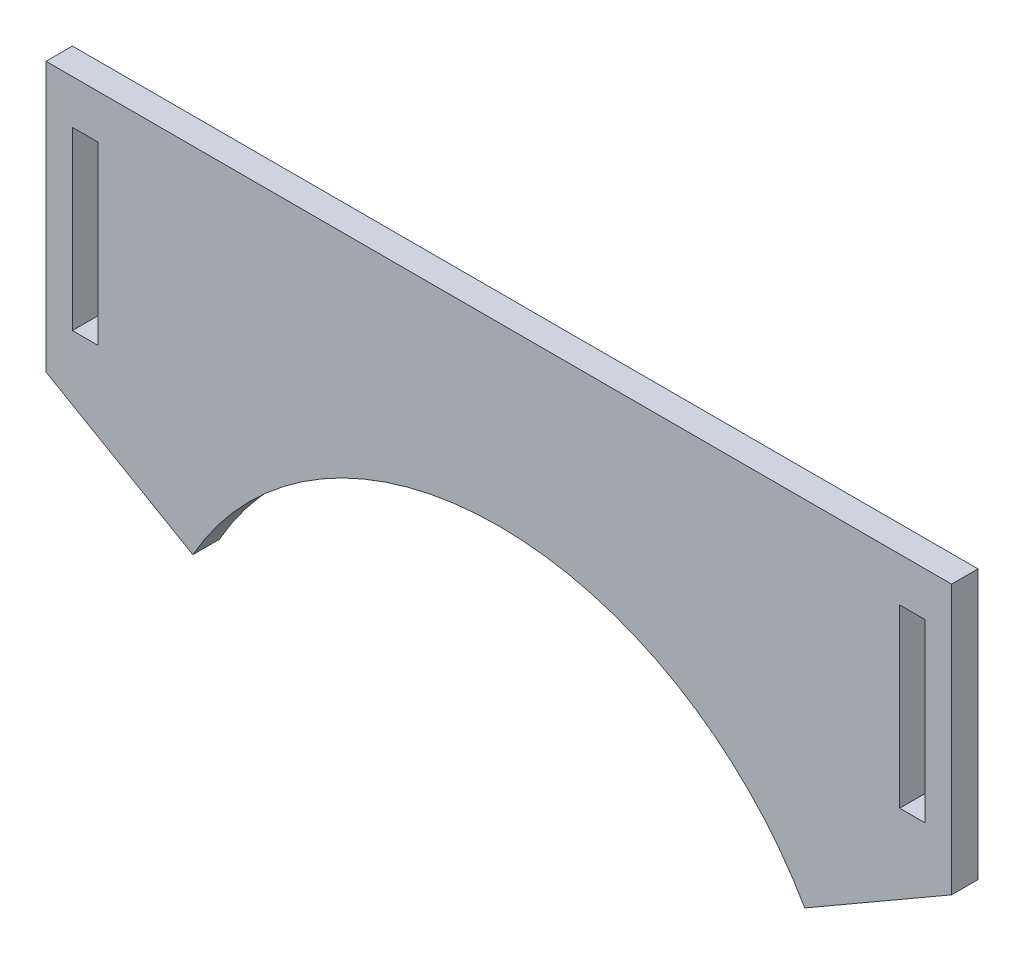
SolidWorks part; units mm, degrees
ref_plane "Front Plane" through (0, 0, 0) normal (0, 0, 1) x (1, 0, 0)
ref_plane "Top Plane" through (0, 0, 0) normal (0, 1, 0) x (1, 0, 0)
ref_plane "Right Plane" through (0, 0, 0) normal (1, 0, 0) x (0, 0, -1)
sketch "Sketch1" plane through (0, 0, 0) normal (0, 0, 1) x (1, 0, 0)
  line L1 (0, 0) -> (104.9, 0)
  line L2 (0, 0) -> (0, -30)
  line L4 (104.9, 0) -> (104.9, -30)
  line L6 (0, -30) -> (17.6875, -40.2119)
  line L7 (104.9, -30) -> (87.2125, -40.2119)
  line L13 (98, -5) -> (100.9, -5)
  line L14 (98, -5) -> (98, -25)
  line L15 (98, -25) -> (100.9, -25)
  line L16 (100.9, -5) -> (100.9, -25)
  line L20 (4, -5) -> (6.9, -5)
  line L21 (4, -5) -> (4, -25)
  line L22 (4, -25) -> (6.9, -25)
  line L23 (6.9, -5) -> (6.9, -25)
  line L26 (52.45, -20) -> (52.45, 0) construction
  arc A0 (87.2125, -40.2119) -> (17.6875, -40.2119) centre (52.45, -60) ccw
  dimension "D1" = 20
  dimension "D4" = 5
  dimension "D7" = 40
  dimension "D2" = 2.9
  dimension "D3" = 4
  dimension "D5" = 30
  dimension "D6" = 2.9
  dimension "D8" = 94
  dimension "D9" = 4
  dimension "D10" = 60
  dimension "D11" = 52.45
  dimension "D12" = 120
  dimension "D13" = 120
  dimension "D14" = 30
extrude "Boss-Extrude1" add sketch "Sketch1" along normal blind 3
sketch "Sketch2" plane through (0, 0, 3) normal (0, 0, 1) x (1, 0, 0)
  line L0 (1, 0) -> (1, -30.5774)
  line L1 (104.9, 0) -> (0, 0) construction
  line L2 (0, -30) -> (17.6875, -40.2119) construction
  line L3 (0, 0) -> (0, -30) construction
  line L4 (103.9, 0) -> (103.9, -30.5774)
  line L5 (87.2125, -40.2119) -> (104.9, -30) construction
  line L6 (104.9, -30) -> (104.9, 0) construction
  line L7 (1, 0) -> (0, 0)
  line L8 (0, 0) -> (0, -30)
  line L9 (0, -30) -> (1, -30.5774)
  line L11 (103.9, -30.5774) -> (104.9, -30)
  line L12 (104.9, -30) -> (104.9, 0)
  line L13 (104.9, 0) -> (103.9, 0)
  dimension "D1" = 1
  dimension "D2" = 1
extrude "Cut-Extrude1" cut sketch "Sketch2" against normal through all
